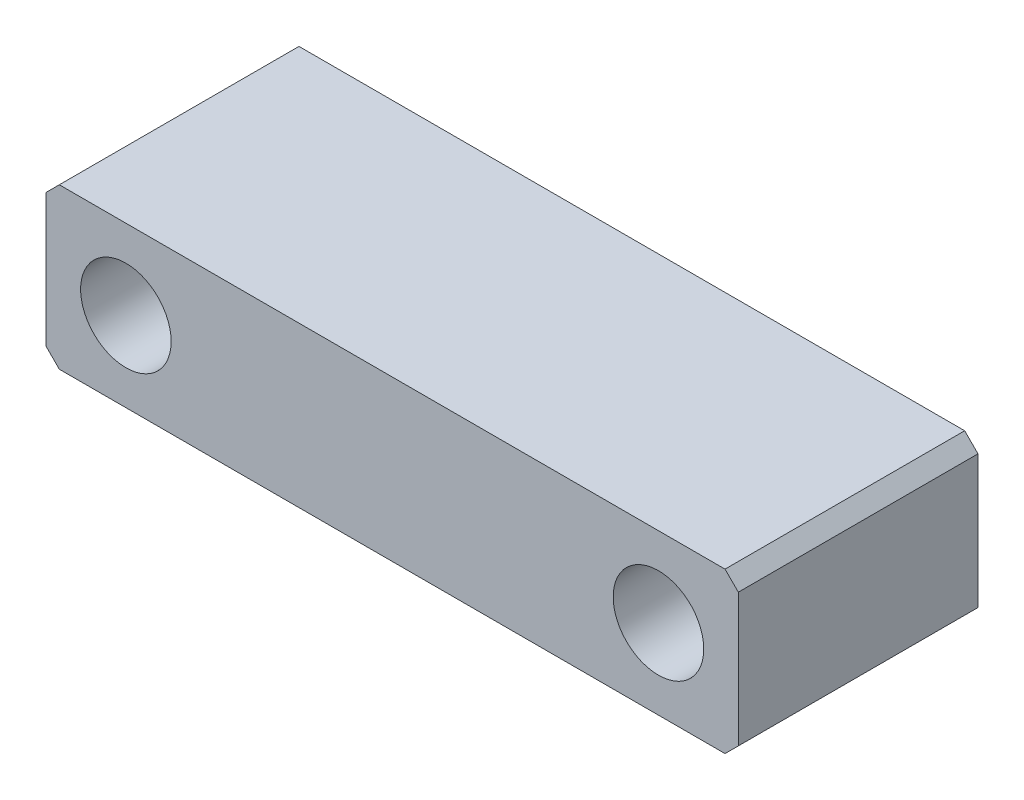
from build123d import *

# Parameters (mm, degrees)
SKETCH1_W                = 26
SKETCH1_H                = 6
BOSS_EXTRUDE1_DEPTH      = 9
M3_CLEARANCE_HOLE1_D     = 3.4
M3_CLEARANCE_HOLE1_DEPTH = 30
M3_CLEARANCE_HOLE1_TIP   = 1.021463052
CHAMFER1_SIZE            = 0.5


with BuildPart() as part:
    # Sketch1 → Boss-Extrude1 (new body)
    with BuildSketch(Plane.XY):
        Rectangle(SKETCH1_W, SKETCH1_H)
    extrude(amount=BOSS_EXTRUDE1_DEPTH)

    # M3 Clearance Hole1
    with Locations(Plane.XY.offset(9)):
        with Locations((-10, 0), (10, 0)):
            Hole(M3_CLEARANCE_HOLE1_D / 2, depth=M3_CLEARANCE_HOLE1_DEPTH)
            with Locations((0, 0, -(M3_CLEARANCE_HOLE1_DEPTH + M3_CLEARANCE_HOLE1_TIP / 2))):  # 118° drill point
                Cone(0, M3_CLEARANCE_HOLE1_D / 2, M3_CLEARANCE_HOLE1_TIP, mode=Mode.SUBTRACT)

    # Chamfer1
    chamfer1_edges = [part.edges().sort_by_distance(p)[0] for p in [
        (13, -3, 4.5),
        (-13, -3, 4.5),
        (-13, 3, 4.5),
        (13, 3, 4.5),
    ]]
    chamfer(chamfer1_edges, length=CHAMFER1_SIZE)


solid = part.part
